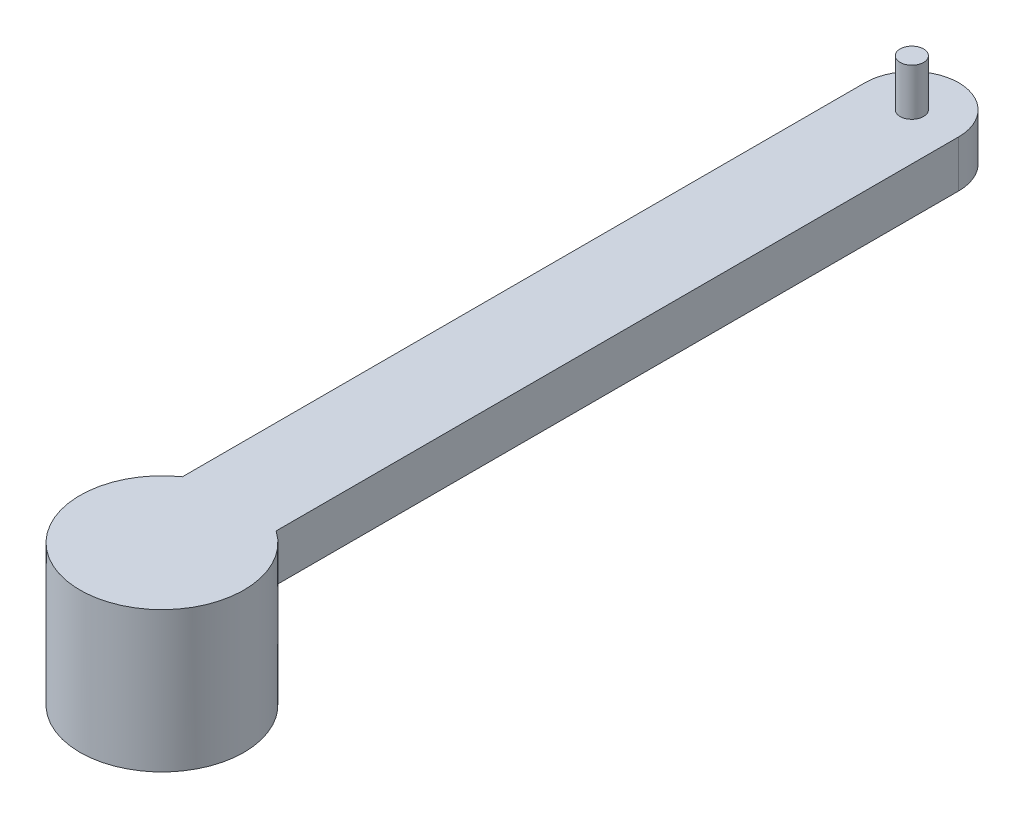
SolidWorks part; units mm, degrees
ref_plane "前视" through (0, 0, 0) normal (0, 0, 1) x (1, 0, 0)
ref_plane "上视" through (0, 0, 0) normal (0, 1, 0) x (1, 0, 0)
ref_plane "右视" through (0, 0, 0) normal (1, 0, 0) x (0, 0, -1)
sketch "草图1" plane through (0, 0, 0) normal (0, 1, 0) x (1, 0, 0)
  circle A0 centre (0, 0) radius 17.5
extrude "凸台-拉伸1" add sketch "草图1" along normal blind 30
sketch "草图2" plane through (0, 0, 0) normal (0, -1, 0) x (1, 0, 0)
  circle A0 centre (0, 0) radius 5
extrude "切除-拉伸1" cut sketch "草图2" against normal blind 24
sketch "草图3" plane through (0, 30, 0) normal (0, 1, 0) x (1, 0, 0)
  line L0 (0, 0) -> (0, 170) construction
  line L2 (-10, 160) -> (-10, 0)
  line L3 (-10, 0) -> (10, 0)
  line L4 (10, 160) -> (10, 0)
  arc A1 (10, 160) -> (-10, 160) centre (0, 160) ccw
  dimension "D1" = 160
extrude "凸台-拉伸2" add sketch "草图3" against normal blind 10
sketch "草图4" plane through (0, 30, 0) normal (0, 1, 0) x (1, 0, 0)
  line L0 (-10, 160) -> (-10, 14.3614) construction
  circle A0 centre (0, 160) radius 2.5
  arc A1 (10, 160) -> (-10, 160) centre (0, 160) ccw construction
  point P2 (0, 170)
  dimension "D1" = 5
  dimension "D2" = 10
  dimension "D3" = 10
extrude "凸台-拉伸3" add sketch "草图4" along normal blind 10
